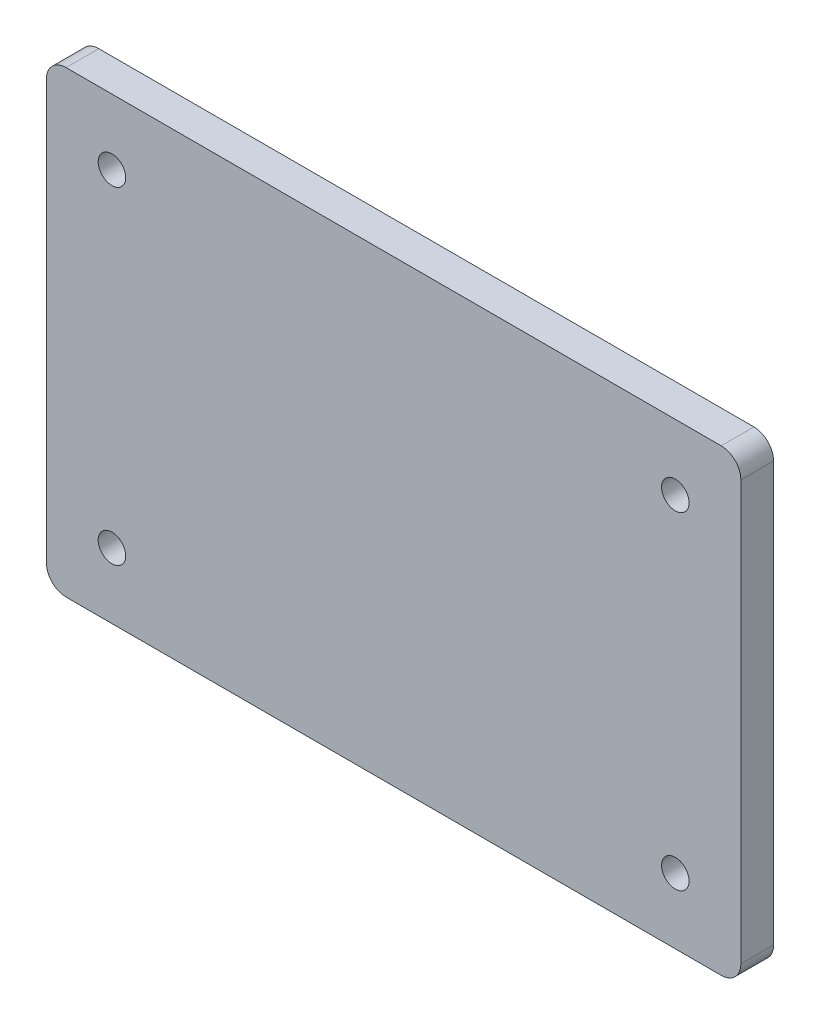
SolidWorks part; units mm, degrees
ref_plane "前视基准面" through (0, 0, 0) normal (0, 0, 1) x (1, 0, 0)
ref_plane "上视基准面" through (0, 0, 0) normal (0, 1, 0) x (1, 0, 0)
ref_plane "右视基准面" through (0, 0, 0) normal (1, 0, 0) x (0, 0, -1)
sketch "草图1" plane through (0, 0, 0) normal (0, 0, 1) x (1, 0, 0)
  line L1 (-53, 35) -> (53, 35)
  line L2 (-53, 35) -> (-53, -35)
  line L3 (-53, -35) -> (53, -35)
  line L4 (53, 35) -> (53, -35)
  line L5 (0, -35) -> (0, 35) construction
  line L6 (-53, 0) -> (53, 0) construction
  point P0 (0, 0)
  dimension "D1" = 106
  dimension "D2" = 70
extrude "凸台-拉伸1" add sketch "草图1" along normal mid plane 5
sketch "草图2" plane through (0, 0, 2.5) normal (0, 0, 1) x (1, 0, 0)
  line L0 (0, 0) -> (0, 35) construction
  line L1 (53, 35) -> (-53, 35) construction
  line L2 (0, 0) -> (-53, 0) construction
  line L3 (-53, 35) -> (-53, -35) construction
  circle A0 centre (-43, 25) radius 2.1
  circle A1 centre (43, 25) radius 2.1
  circle A2 centre (43, -25) radius 2.1
  circle A3 centre (-43, -25) radius 2.1
  dimension "D1" = 4.2
  dimension "D2" = 86
  dimension "D3" = 50
extrude "切除-拉伸1" cut sketch "草图2" against normal through all
fillet "圆角1" radius 3 4 edges at (-53, -35, 0) (53, -35, 0) (53, 35, 0) (-53, 35, 0)
